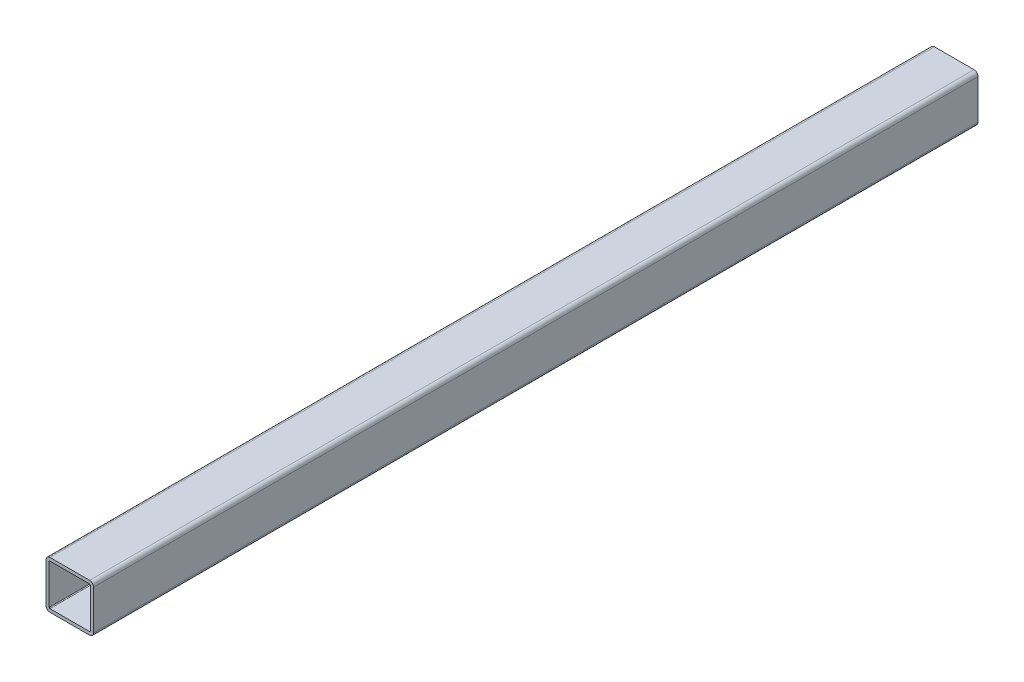
SolidWorks part; units mm, degrees
material "1023 碳钢板 (SS)"
ref_plane "Front Plane" through (0, 0, 0) normal (0, 0, 1) x (1, 0, 0)
ref_plane "Top Plane" through (0, 0, 0) normal (0, 1, 0) x (1, 0, 0)
ref_plane "Right Plane" through (0, 0, 0) normal (1, 0, 0) x (0, 0, -1)
sketch "Sketch1" plane through (0, 0, 0) normal (0, 0, 1) x (1, 0, 0)
  line L1 (30, 30) -> (-30, 30)
  line L2 (30, 30) -> (30, -30)
  line L3 (30, -30) -> (-30, -30)
  line L4 (-30, 30) -> (-30, -30)
  line L5 (30, 30) -> (-30, -30) construction
  line L6 (30, -30) -> (-30, 30) construction
  point P0 (0, 0)
  dimension "D1" = 60
  dimension "D2" = 60
extrude "Boss-Extrude1" add sketch "Sketch1" along normal blind 1116 contours L2 L1 L4 L3
fillet "Fillet1" radius 5 4 edges at (-30, 30, 558) (30, 30, 558) (30, -30, 558) (-30, -30, 558)
shell "Shell1" thickness 4
